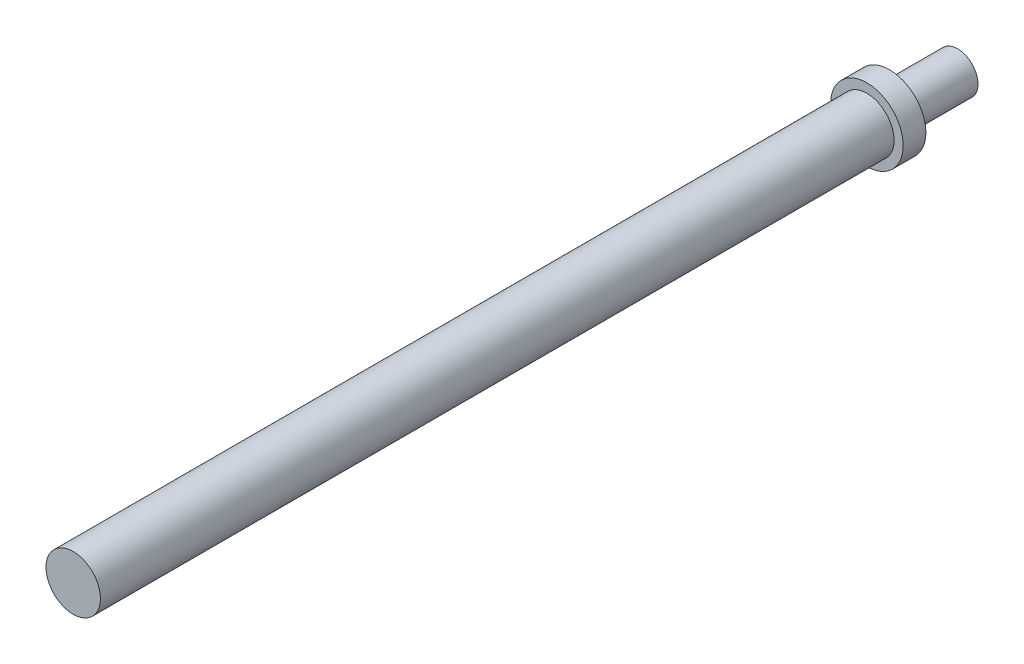
SolidWorks part; units mm, degrees
ref_plane "前视基准面" through (0, 0, 0) normal (0, 0, 1) x (1, 0, 0)
ref_plane "上视基准面" through (0, 0, 0) normal (0, 1, 0) x (1, 0, 0)
ref_plane "右视基准面" through (0, 0, 0) normal (1, 0, 0) x (0, 0, -1)
sketch "草图1" plane through (0, 0, 0) normal (0, 0, 1) x (1, 0, 0)
  circle A0 centre (0, 0) radius 4.5
  dimension "D1" = 9
extrude "凸台-拉伸1" add sketch "草图1" along normal blind 15
cosmetic thread "装饰螺纹线1" parameters "D1"=15, "D2"=8
sketch "草图2" plane through (0, 0, 15) normal (0, 0, 1) x (1, 0, 0)
  circle A0 centre (0, 0) radius 6
  dimension "D1" = 12
extrude "凸台-拉伸2" add sketch "草图2" along normal blind 180
sketch "草图3" plane through (0, 0, 15) normal (0, 0, -1) x (-1, 0, 0)
  circle A0 centre (0, 0) radius 8
  dimension "D1" = 16
extrude "凸台-拉伸3" add sketch "草图3" against normal blind 5
